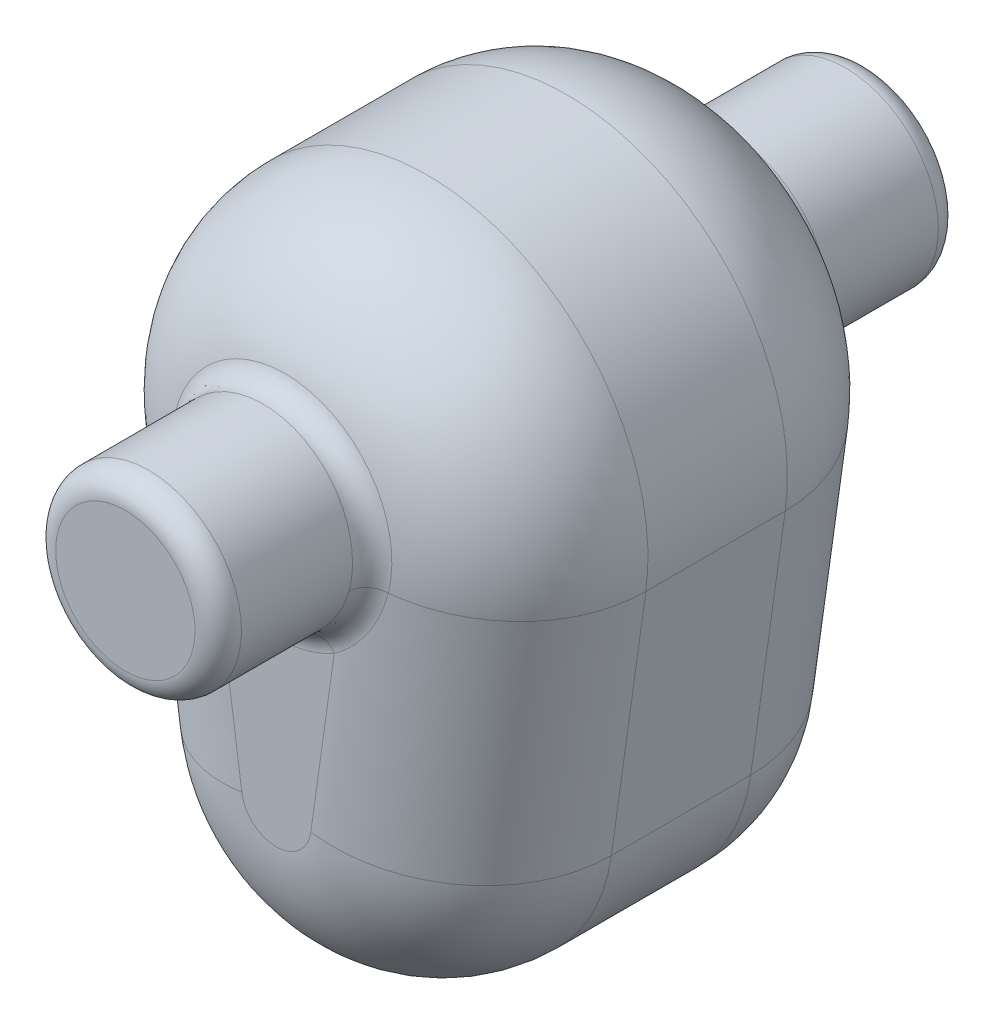
from build123d import *

# Parameters (mm, degrees)
BOSS_EXTRUDE1_DEPTH = 19
FILLET1_R           = 6.5
SKETCH2_R           = 4
BOSS_EXTRUDE2_DEPTH = 16
FILLET2_R           = 1
FILLET4_R           = 1


with BuildPart() as part:
    # Sketch1 → Boss-Extrude1 (new body)
    with BuildSketch(Plane.XY):
        with BuildLine():
            Line((-15.01441447, -2.268498309), (-13.528952514, -12.860164976))
            ThreePointArc((-13.528952514, -12.860164976), (-5.606488749, -19.749053865), (2.315975015, -12.860164976))
            Line((2.315975015, -12.860164976), (3.801436971, -2.268498309))
            ThreePointArc((3.801436971, -2.268498309), (-5.606488749, 8.550946135), (-15.01441447, -2.268498309))
        make_face()
    extrude(amount=BOSS_EXTRUDE1_DEPTH)

    # Fillet1
    fillet1_edges = [part.edges().sort_by_distance(p)[0] for p in [
        (-5.606488749, 8.550946135, 19),
        (-14.271683492, -7.564331643, 19),
        (-5.606488749, -19.749053865, 19),
        (-14.271683492, -7.564331643, 0),
        (-5.606488749, 8.550946135, 0),
        (3.058705993, -7.564331643, 0),
        (-5.606488749, -19.749053865, 0),
        (3.058705993, -7.564331643, 19),
    ]]
    fillet(fillet1_edges, radius=FILLET1_R)

    # Sketch2 → Boss-Extrude2 (add, symmetric)
    with BuildSketch(Plane.XY.offset(9.5)):
        with Locations(Location((-5.606488749, -0.449053865, 0), (0, 0, 195.094354514))):
            Circle(SKETCH2_R)
    extrude(amount=BOSS_EXTRUDE2_DEPTH, both=True)

    # Fillet2
    fillet2_edges = [part.edges().sort_by_distance(p)[0] for p in [
        (-1.744495572, 0.592583644, -6.5),
        (-1.744495572, 0.592583644, 25.5),
    ]]
    fillet(fillet2_edges, radius=FILLET2_R)

    # Fillet4
    fillet4_edges = [part.edges().sort_by_distance(p)[0] for p in [
        (-2.195166372, -2.537804614, 18.972348526),
        (-5.606488749, -4.449053865, 0),
        (-2.195166372, -2.537804614, 0.027651474),
        (-5.606488749, 3.550946135, 0.17544468),
        (-9.017811127, -2.537804614, 0.027651474),
        (-5.606488749, -4.449053865, 19),
        (-9.017811127, -2.537804614, 18.972348526),
        (-5.606488749, 3.550946135, 18.82455532),
    ]]
    fillet(fillet4_edges, radius=FILLET4_R)


solid = part.part
